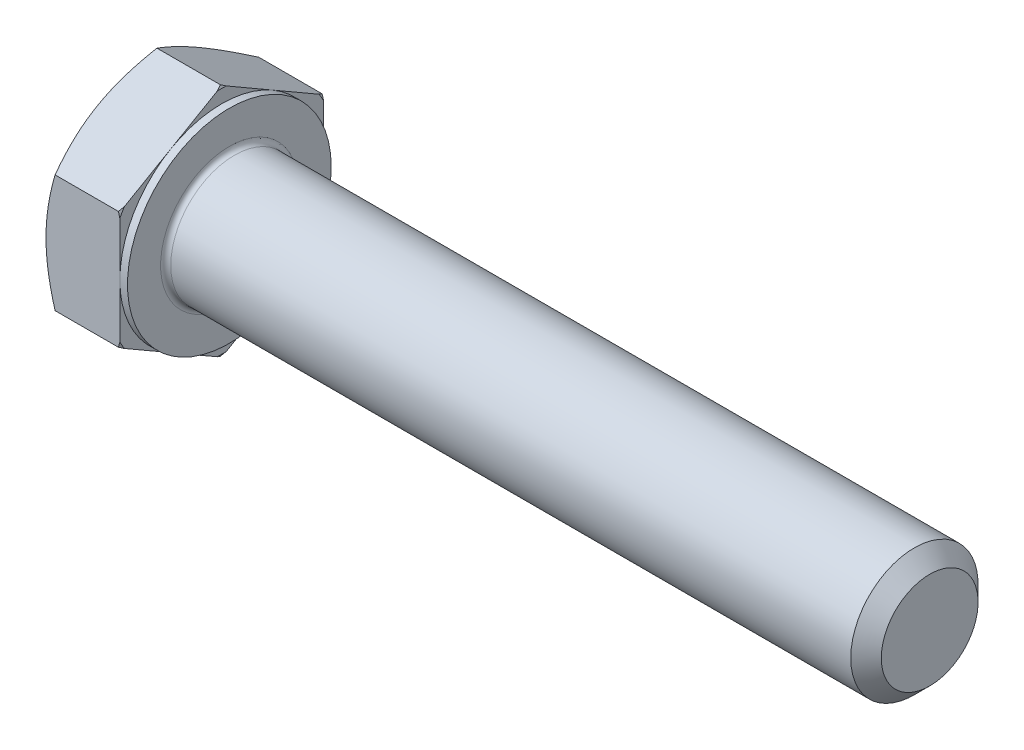
from build123d import *

# Parameters (mm, degrees)
EXTRUDE_371_DEPTH = 6.4
SKETCH_4_W        = 0.6
SKETCH_4_H        = 11.237604307
CHAMFER_2038_SIZE = 1.2
FILLET_2080_R     = 0.4


with BuildPart() as part:
    # 草图1 → Extrude 371 (new body)
    with BuildSketch(Plane(origin=(0, 0, 0), x_dir=(0, 0, -1), z_dir=(1, 0, 0))):
        Polygon((8, 4.618802154), (8, -4.618802154), (0, -9.237604307), (-8, -4.618802154), (-8, 4.618802154), (0, 9.237604307), align=None)
    extrude(amount=EXTRUDE_371_DEPTH)

    # 草图2 → 凸台-旋转1 (revolve)
    with BuildSketch(Plane.XY, mode=Mode.PRIVATE) as revolve_1_sk:
        Polygon((0, 0), (61.4, 0), (61.4, 3.701), (61.4, 5), (27.8072, 5), (0, 5), align=None)
    revolve(revolve_1_sk.sketch.rotate(Axis((0, 0, 0), (1, 0, 0)), 90), axis=Axis((0, 0, 0), (1, 0, 0)))

    # 草图3 → 切除-旋转1 (revolve, cut)
    with BuildSketch(Plane.XY):
        Polygon((0, 8), (3.601282526, 14.237604307), (3.601282526, 19.237604307), (-10, 19.237604307), (-10, 8), align=None)
    revolve(axis=Axis((0, 0, 0), (1, 0, 0)), mode=Mode.SUBTRACT)

    # 草图5 → 切除-旋转2 (revolve, cut)
    with BuildSketch(Plane.XY):
        Polygon((6.4, 8), (2.798717474, 14.237604307), (2.798717474, 19.237604307), (12.798717474, 19.237604307), (12.798717474, 8), align=None)
    revolve(axis=Axis((0, 0, 0), (1, 0, 0)), mode=Mode.SUBTRACT)

    # 草图4 → 切除-旋转3 (revolve, cut)
    with BuildSketch(Plane.XY, mode=Mode.PRIVATE) as cut_revolve_3_sk:
        with Locations((6.1, 13.618802154)):
            Rectangle(SKETCH_4_W, SKETCH_4_H)
    revolve(cut_revolve_3_sk.sketch.rotate(Axis((0, 0, 0), (1, 0, 0)), 270), axis=Axis((0, 0, 0), (1, 0, 0)), mode=Mode.SUBTRACT)

    # Chamfer 2038
    chamfer_2038_edges = [part.edges().sort_by_distance(p)[0] for p in [
        (61.4, 0, -5),
    ]]
    chamfer(chamfer_2038_edges, length=CHAMFER_2038_SIZE)

    # Fillet 2080
    fillet_2080_edges = [part.edges().sort_by_distance(p)[0] for p in [
        (6.4, 0, -5),
    ]]
    fillet(fillet_2080_edges, radius=FILLET_2080_R)


solid = part.part
